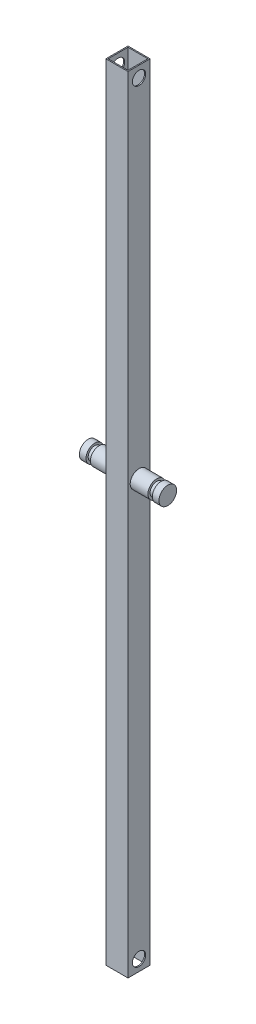
from build123d import *

# Parameters (mm, degrees)
SKETCH1_W           = 10
SKETCH1_H           = 10
SKETCH1_W_2         = 9
SKETCH1_H_2         = 9
BOSS_EXTRUDE1_DEPTH = 355
SKETCH2_R           = 4
BOSS_EXTRUDE2_DEPTH = 8
SKETCH3_R           = 3
BOSS_EXTRUDE3_DEPTH = 2
SKETCH4_R           = 4
BOSS_EXTRUDE4_DEPTH = 3
SKETCH5_R           = 3
CUT_EXTRUDE1_DEPTH  = 21
SKETCH6_R           = 3
CUT_EXTRUDE2_DEPTH  = 18


with BuildPart() as part:
    # Sketch1 → Boss-Extrude1 (new body)
    with BuildSketch(Plane(origin=(0, 0, 0), x_dir=(1, 0, 0), z_dir=(0, 1, 0))):
        Rectangle(SKETCH1_W, SKETCH1_H)
        Rectangle(SKETCH1_W_2, SKETCH1_H_2, mode=Mode.SUBTRACT)
    extrude(amount=BOSS_EXTRUDE1_DEPTH)

    # Sketch2 → Boss-Extrude2 (add)
    with BuildSketch(Plane(origin=(5, 0, 0), x_dir=(0, 0, -1), z_dir=(1, 0, 0))):
        with Locations(Location((0, 193, 0), (0, 0, 180))):
            Circle(SKETCH2_R)
    extrude(amount=BOSS_EXTRUDE2_DEPTH)

    # Sketch3 → Boss-Extrude3 (add)
    with BuildSketch(Plane(origin=(13, 0, 0), x_dir=(0, 0, -1), z_dir=(1, 0, 0))):
        with Locations((0, 193)):
            Circle(SKETCH3_R)
    extrude(amount=BOSS_EXTRUDE3_DEPTH)

    # Sketch4 → Boss-Extrude4 (add)
    with BuildSketch(Plane(origin=(15, 0, 0), x_dir=(0, 0, -1), z_dir=(1, 0, 0))):
        with Locations(Location((0, 193, 0), (0, 0, 180))):
            Circle(SKETCH4_R)
    extrude(amount=BOSS_EXTRUDE4_DEPTH)

    # Mirror1: part across plane


with BuildPart() as part_1:
    add(part.part)
    add(part.part.mirror(Plane(origin=(0, 0, 0), x_dir=(0, 0, 1), z_dir=(1, 0, 0))))

    # Sketch5 → Cut-Extrude1 (cut)
    with BuildSketch(Plane(origin=(5, 0, 0), x_dir=(0, 0, -1), z_dir=(1, 0, 0))):
        with Locations((0, 5)):
            Circle(SKETCH5_R)
    extrude(amount=-CUT_EXTRUDE1_DEPTH, mode=Mode.SUBTRACT)

    # Sketch6 → Cut-Extrude2 (cut)
    with BuildSketch(Plane.ZY.offset(5)):
        with Locations((0, 350)):
            Circle(SKETCH6_R)
    extrude(amount=-CUT_EXTRUDE2_DEPTH, mode=Mode.SUBTRACT)


solid = part_1.part
